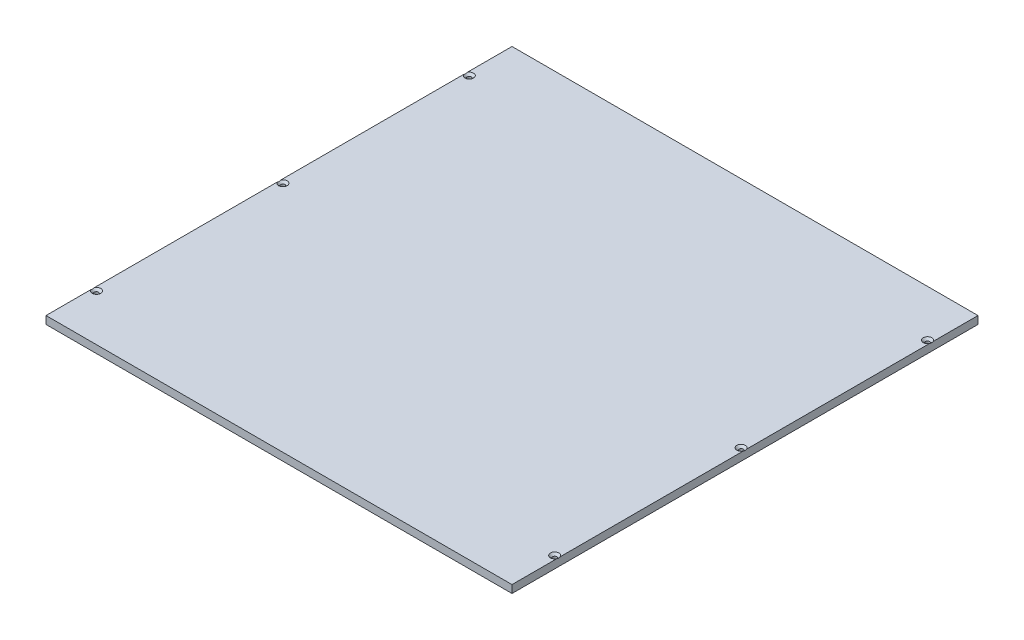
from build123d import *

# Parameters (mm, degrees)
SKETCH1_W                                         = 300
SKETCH1_H                                         = 300
BOSS_EXTRUDE1_DEPTH                               = 5
CSK_FOR_M2_5_FLAT_HEAD_MACHINE_SCREW1_D           = 2.7
CSK_FOR_M2_5_FLAT_HEAD_MACHINE_SCREW1_DEPTH       = 17
CSK_FOR_M2_5_FLAT_HEAD_MACHINE_SCREW1_CSINK_D     = 5.5
CSK_FOR_M2_5_FLAT_HEAD_MACHINE_SCREW1_CSINK_ANGLE = 90
CSK_FOR_M2_5_FLAT_HEAD_MACHINE_SCREW1_TIP         = 0.811161836


with BuildPart() as part:
    # Sketch1 → Boss-Extrude1 (new body)
    with BuildSketch(Plane(origin=(0, 0, 0), x_dir=(1, 0, 0), z_dir=(0, 1, 0))):
        Rectangle(SKETCH1_W, SKETCH1_H)
    extrude(amount=BOSS_EXTRUDE1_DEPTH)

    # CSK for M2.5 Flat Head Machine Screw1
    with Locations(Plane(origin=(0, 5, 0), x_dir=(1, 0, 0), z_dir=(0, 1, 0))):
        with Locations((147.5, 120), (147.5, 0), (147.5, -120), (-147.5, 120), (-147.5, 0), (-147.5, -120)):
            CounterSinkHole(CSK_FOR_M2_5_FLAT_HEAD_MACHINE_SCREW1_D / 2, CSK_FOR_M2_5_FLAT_HEAD_MACHINE_SCREW1_CSINK_D / 2, depth=CSK_FOR_M2_5_FLAT_HEAD_MACHINE_SCREW1_DEPTH, counter_sink_angle=CSK_FOR_M2_5_FLAT_HEAD_MACHINE_SCREW1_CSINK_ANGLE)
            with Locations((0, 0, -(CSK_FOR_M2_5_FLAT_HEAD_MACHINE_SCREW1_DEPTH + CSK_FOR_M2_5_FLAT_HEAD_MACHINE_SCREW1_TIP / 2))):  # 118° drill point
                Cone(0, CSK_FOR_M2_5_FLAT_HEAD_MACHINE_SCREW1_D / 2, CSK_FOR_M2_5_FLAT_HEAD_MACHINE_SCREW1_TIP, mode=Mode.SUBTRACT)


solid = part.part
